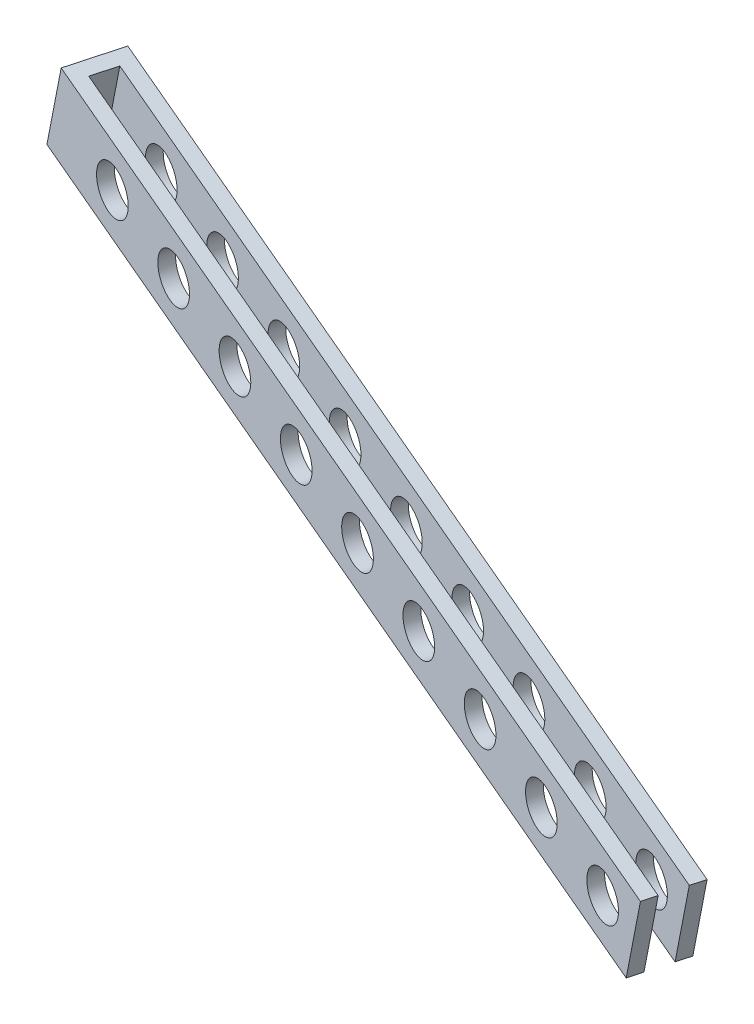
SolidWorks part; units mm, degrees
ref_plane "Front Plane" through (0, 0, 0) normal (0, 0, 1) x (1, 0, 0)
ref_plane "Top Plane" through (0, 0, 0) normal (0, 1, 0) x (1, 0, 0)
ref_plane "Right Plane" through (0, 0, 0) normal (1, 0, 0) x (0, 0, -1)
ref_plane "Plane4" through (-52.0152, 0, 189.7737) normal (-0.2643, 0, 0.9644) x (0.9644, 0, 0.2643)
sketch "Sketch1" plane through (-52.0152, 0, 189.7737) normal (-0.2643, 0, 0.9644) x (0.9644, 0, 0.2643)
  line L0 (31.2675, 172.8773) -> (457.1463, 62.9849)
  line L3 (31.2675, 172.8773) -> (-0.4674, 181.0661)
extrude "Extrude-Thin1" add sketch "Sketch1" against normal up to surface (15 mm away) and the other way up to surface (15 mm away) thin thin type mid plane wall 45
sketch "Sketch2" plane through (-55.9803, 0, 204.2402) normal (-0.2643, 0, 0.9644) x (0.9644, 0, 0.2643)
  line L0 (457.1463, 62.9849) -> (-0.4674, 181.0661) construction
  line L1 (462.768, 84.7713) -> (451.5246, 41.1986) construction
  line L2 (-6.0891, 159.2797) -> (5.1543, 202.8525) construction
  circle A0 centre (432.9392, 69.2313) radius 12.5
  circle A1 centre (384.525, 81.7239) radius 12.5
  circle A2 centre (336.1109, 94.2165) radius 12.5
  circle A3 centre (287.6967, 106.7092) radius 12.5
  circle A4 centre (239.2825, 119.2018) radius 12.5
  circle A5 centre (190.8683, 131.6945) radius 12.5
  circle A6 centre (142.4541, 144.1871) radius 12.5
  circle A7 centre (94.0399, 156.6797) radius 12.5
  circle A8 centre (45.6257, 169.1724) radius 12.5
  dimension "D1" = 25
  dimension "D2" = 25
  dimension "D3" = 9
extrude "Cut-Extrude1" cut sketch "Sketch2" against normal blind 52
sketch "Sketch3" plane through (47.6404, 191.4361, 13.0578) normal (0.241, 0.9683, 0.066) x (0.9705, -0.2404, -0.0164)
  line L4 (361.2616, -291.177) -> (353.0906, -320.0428) construction
  line L6 (359.0827, -298.8745) -> (355.2696, -312.3452)
  line L8 (347.572, -310.1663) -> (351.3851, -296.6956)
  line L9 (351.3851, -296.6956) -> (-87.9552, -172.3323)
  line L10 (-87.9552, -172.3323) -> (-91.7683, -185.803)
  line L11 (-91.7683, -185.803) -> (347.572, -310.1663)
  line L13 (359.0827, -298.8745) -> (-87.9552, -172.3323)
  line L14 (-87.9552, -172.3323) -> (-91.7683, -185.803)
  line L15 (-91.7683, -185.803) -> (355.2696, -312.3452)
  dimension "D1" = 8
extrude "Cut-Extrude2" cut sketch "Sketch3" against normal blind 52
